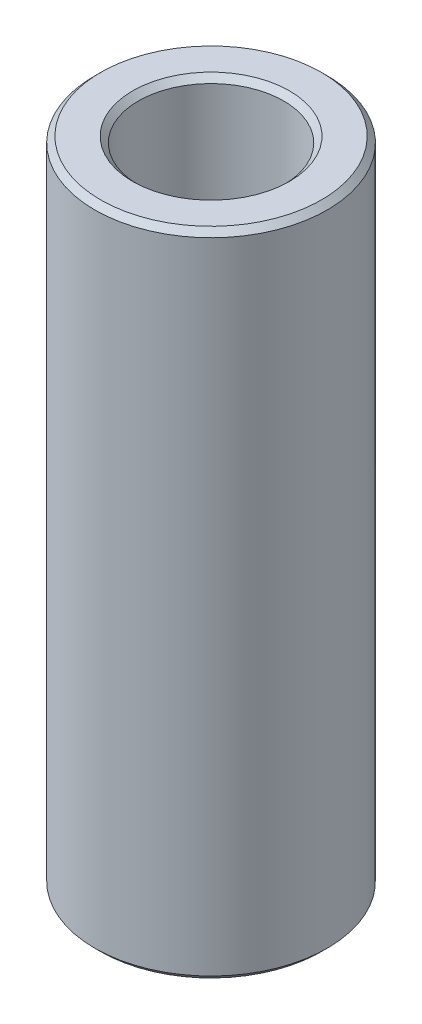
from build123d import *

# Parameters (mm, degrees)
SKETCH1_R           = 20
SKETCH1_R_2         = 12.5
BOSS_EXTRUDE1_DEPTH = 112
CHAMFER1_SIZE       = 1


with BuildPart() as part:
    # Sketch1 → Boss-Extrude1 (new body)
    with BuildSketch(Plane(origin=(0, 0, 0), x_dir=(1, 0, 0), z_dir=(0, 1, 0))):
        with Locations(Location((0, 0, 0), (0, 0, 270))):
            Circle(SKETCH1_R)
        with Locations(Location((0, 0, 0), (0, 0, 270))):
            Circle(SKETCH1_R_2, mode=Mode.SUBTRACT)
    extrude(amount=BOSS_EXTRUDE1_DEPTH)

    # Chamfer1
    chamfer1_edges = [part.edges().sort_by_distance(p)[0] for p in [
        (0, 0, -20),
        (0, 112, -20),
        (0, 0, -12.5),
        (0, 112, -12.5),
    ]]
    chamfer(chamfer1_edges, length=CHAMFER1_SIZE)


solid = part.part
